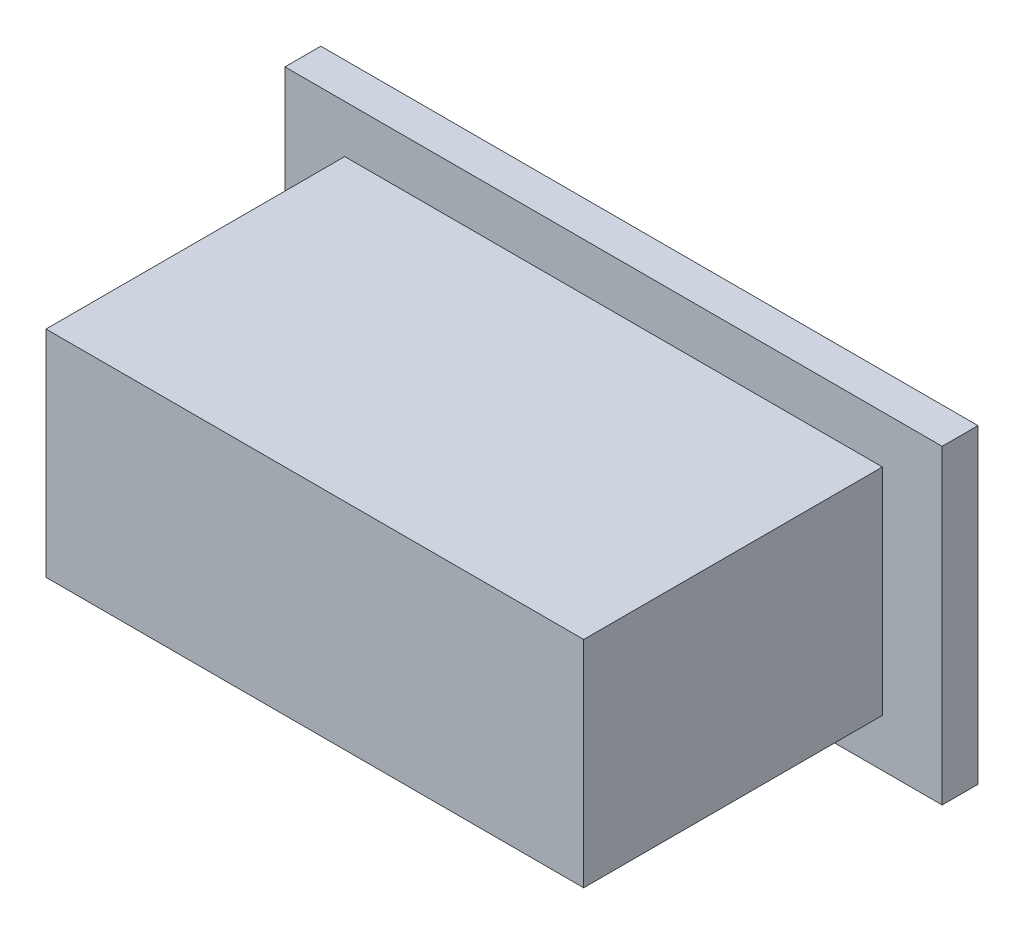
from build123d import *

# Parameters (mm, degrees)
SKETCH1_W                = 450
SKETCH1_H                = 280
BOSS_EXTRUDE1_DEPTH      = 180
BOSS_EXTRUDE2_DEPTH      = 40
BOSS_EXTRUDE2_DEPTH_BACK = 220
SKETCH2_W                = 550
SKETCH2_H                = 30


with BuildPart() as part:
    # Sketch1 → Boss-Extrude1 (new body)
    with BuildSketch(Plane(origin=(0, 0, 0), x_dir=(1, 0, 0), z_dir=(0, 1, 0))):
        with Locations((225, -140)):
            Rectangle(SKETCH1_W, SKETCH1_H)
    extrude(amount=BOSS_EXTRUDE1_DEPTH)

    # Sketch2 → Boss-Extrude2 (add, two sides: drawn at the far end of the back side and taken through both)
    with BuildSketch(Plane.XZ.offset(-BOSS_EXTRUDE2_DEPTH_BACK)):
        with Locations((225, 15)):
            Rectangle(SKETCH2_W, SKETCH2_H)
    extrude(amount=BOSS_EXTRUDE2_DEPTH + BOSS_EXTRUDE2_DEPTH_BACK)


solid = part.part
